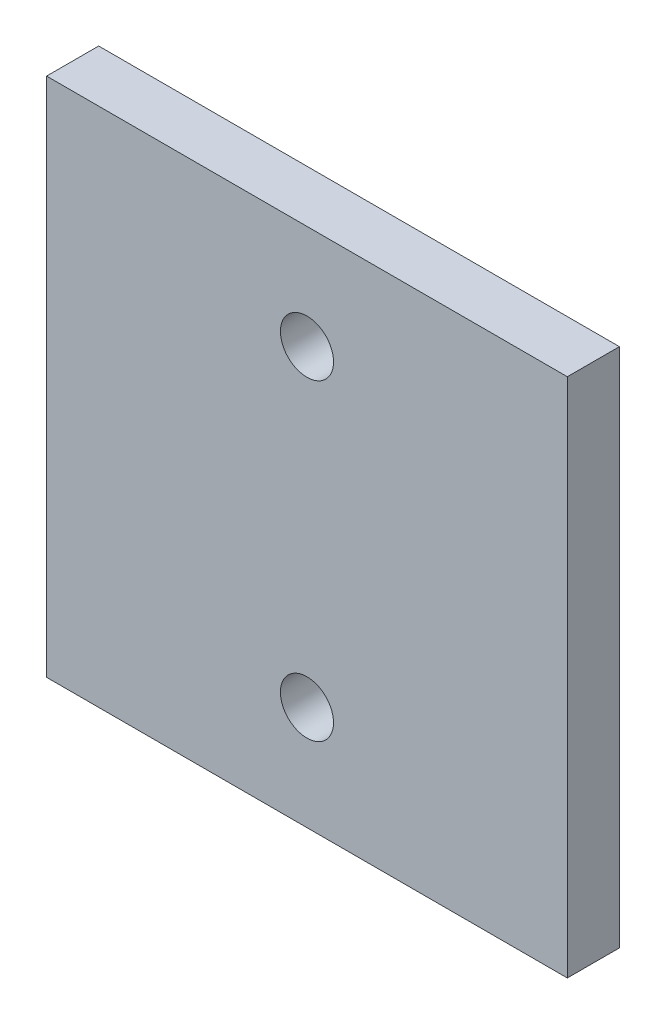
from build123d import *

# Parameters (mm, degrees)
SKETCH1_W              = 100
SKETCH1_H              = 100
BOSS_EXTRUDE1_DEPTH    = 10
M12_TAPPED_HOLE1_D     = 10.2
M12_TAPPED_HOLE1_DEPTH = 29.25
M12_TAPPED_HOLE1_TIP   = 3.064389157


with BuildPart() as part:
    # Sketch1 → Boss-Extrude1 (new body)
    with BuildSketch(Plane.XY):
        Rectangle(SKETCH1_W, SKETCH1_H)
    extrude(amount=BOSS_EXTRUDE1_DEPTH)

    # M12 Tapped Hole1
    with Locations(Plane.XY.offset(10)):
        with Locations((0, 30), (0, -30)):
            Hole(M12_TAPPED_HOLE1_D / 2, depth=M12_TAPPED_HOLE1_DEPTH)
            with Locations((0, 0, -(M12_TAPPED_HOLE1_DEPTH + M12_TAPPED_HOLE1_TIP / 2))):  # 118° drill point
                Cone(0, M12_TAPPED_HOLE1_D / 2, M12_TAPPED_HOLE1_TIP, mode=Mode.SUBTRACT)


solid = part.part
